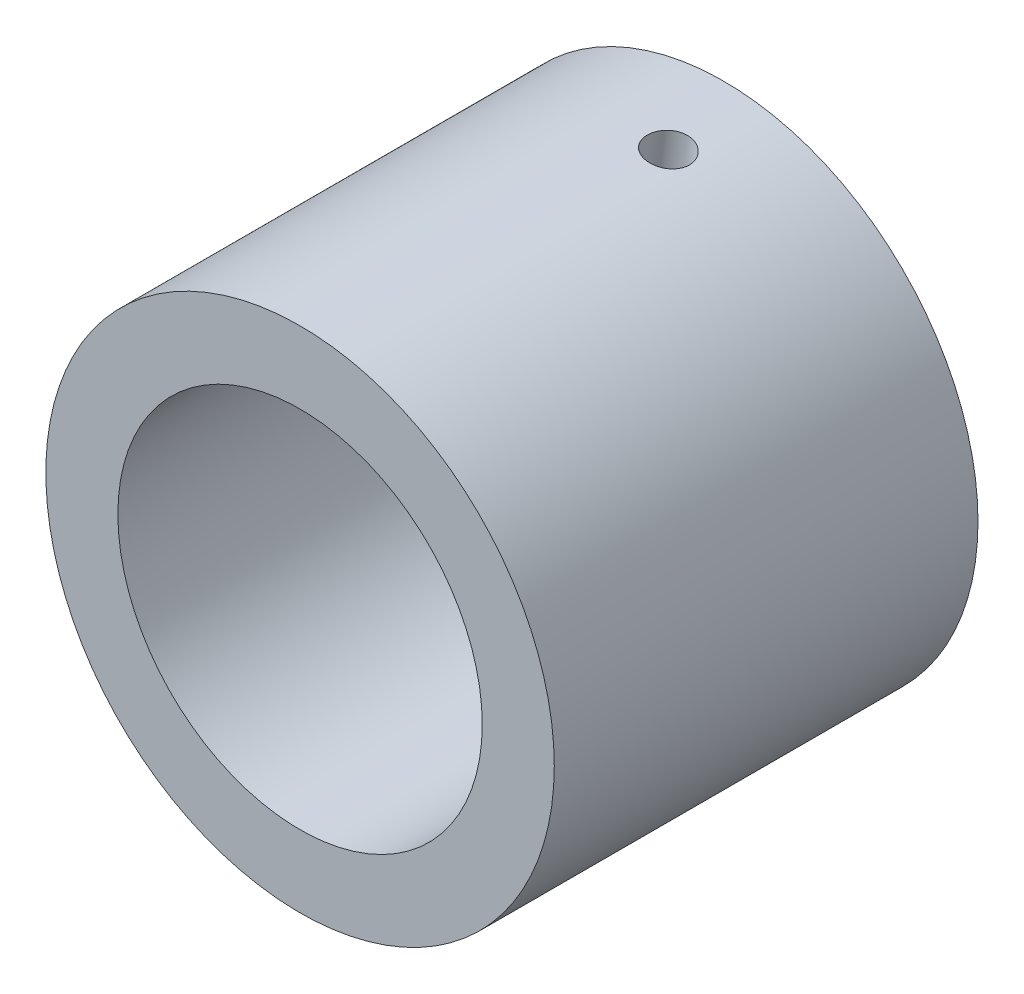
SolidWorks part; units mm, degrees
material "普通碳钢"
ref_plane "Front Plane" through (0, 0, 0) normal (0, 0, 1) x (1, 0, 0)
ref_plane "Top Plane" through (0, 0, 0) normal (0, 1, 0) x (1, 0, 0)
ref_plane "Right Plane" through (0, 0, 0) normal (1, 0, 0) x (0, 0, -1)
sketch "Sketch1" plane through (0, 0, 0) normal (0, 0, 1) x (1, 0, 0)
  circle A0 centre (0, 0) radius 30
  circle A1 centre (0, 0) radius 21.5
  dimension "D1" = 43
  dimension "D2" = 60
extrude "Boss-Extrude1" add sketch "Sketch1" against normal blind 50
hole_wizard "M6 Tapped Hole1" positions "3DSketch2" profile "Sketch3" tap size "M6" standard "GB"
sketch3d "3DSketch2"
  point P0 (3.4711, 29.7985, -40)
  dimension "D1" = 10
sketch "Sketch3" plane through (3.4711, 29.7985, -40) normal (0, 0, 1) x (-0.9933, 0.1157, 0)
  line L0 (0, 0) -> (0, 19.5022)
  line L1 (0, 19.5022) -> (2.5, 18)
  line L2 (2.5, 18) -> (2.5, 0)
  line L5 (2.5, 0) -> (0, 0)
  line L10 (0, 19.5022) -> (-2.5, 18) construction
  line L11 (0, -6.35) -> (0, 107.95) construction
  dimension "螺纹孔钻头直径" = 5
  dimension "螺纹孔钻头深度" = 18
  dimension "导头角度" = 118
cosmetic thread "Tapped hole thread 1" parameters "D1"=8.6458, "D2"=6
sketch "Sketch4" plane through (0, 0, 0) normal (0, 0, 1) x (1, 0, 0)
  circle A0 centre (0, 0) radius 21.5
  circle A1 centre (0, 0) radius 25
  dimension "D1" = 43
  dimension "D2" = 50
extrude "Boss-Extrude2" add sketch "Sketch4" along normal blind 24
sketch "Sketch6" plane through (0, 0, 24) normal (0, 0, 1) x (1, 0, 0)
  circle A2 centre (0, 0) radius 21.5
  circle A3 centre (0, 0) radius 25
  dimension "D1" = 43
  dimension "D2" = 50
extrude "Cut-Extrude1" cut sketch "Sketch6" against normal blind 24
